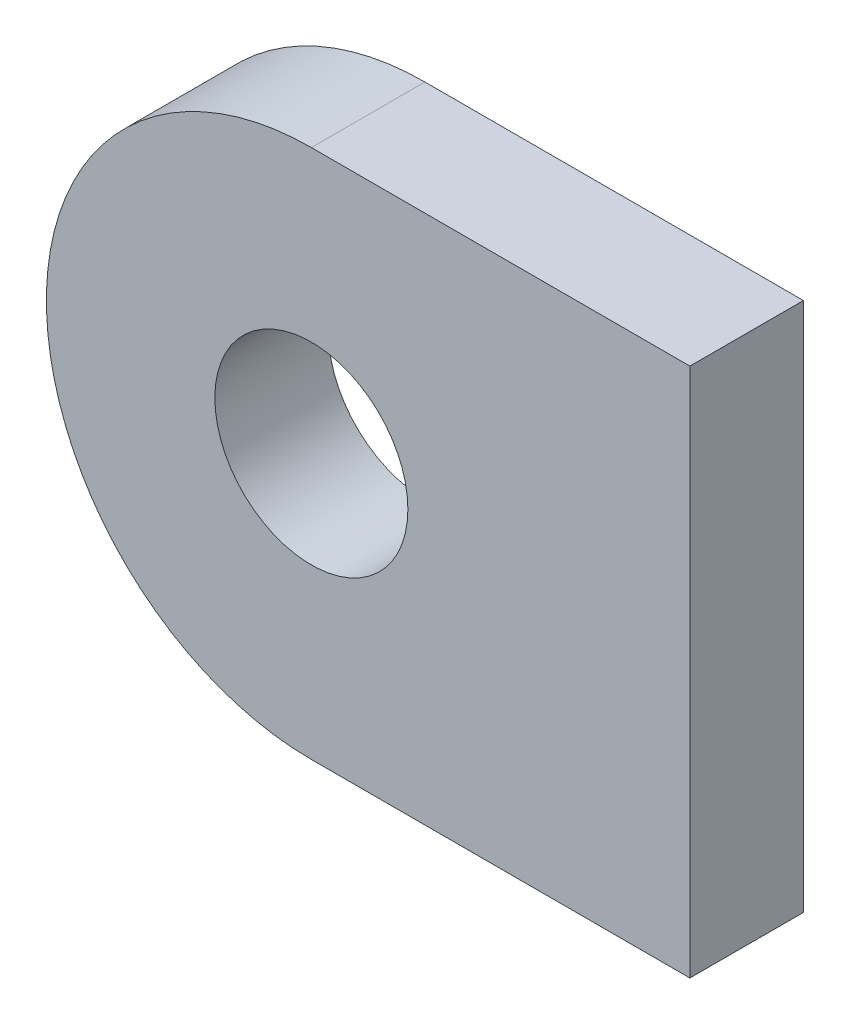
from build123d import *

# Parameters (mm, degrees)
SKETCH_1_R      = 5.1
EXTRUDE_1_DEPTH = 3


with BuildPart() as part:
    # 草图1 → 凸台-拉伸1 (new, symmetric)
    with BuildSketch(Plane.XY):
        with BuildLine():
            Line((0, 14), (20, 14))
            Line((20, 14), (20, -14))
            Line((20, -14), (0, -14))
            ThreePointArc((0, -14), (-14, 0), (0, 14))
        make_face()
        Circle(SKETCH_1_R, mode=Mode.SUBTRACT)
    extrude(amount=EXTRUDE_1_DEPTH, both=True)


solid = part.part
